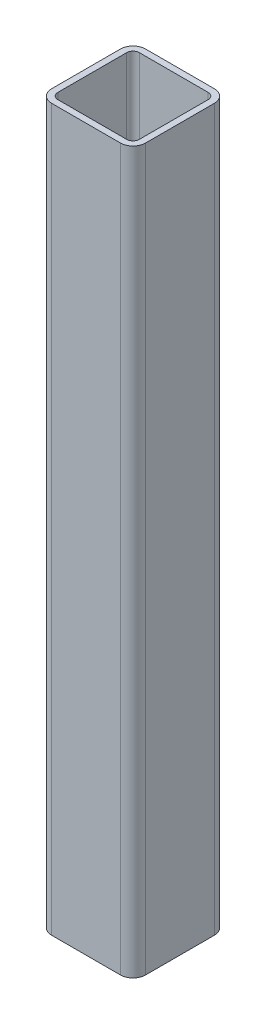
SolidWorks part; units mm, degrees
material "Q235B"
ref_plane "Front Plane" through (0, 0, 0) normal (0, 0, 1) x (1, 0, 0)
ref_plane "Top Plane" through (0, 0, 0) normal (0, 1, 0) x (1, 0, 0)
ref_plane "Right Plane" through (0, 0, 0) normal (1, 0, 0) x (0, 0, -1)
sketch "Sketch1" plane through (0, 0, 0) normal (0, 0, 1) x (1, 0, 0)
  line L0 (0, 0) -> (0, 230)
  dimension "D1" = 230
other "Gb／t 6728—2002 square hollow section 30×30×2(1)"
ref_plane "Plane1" through (0, 0, 0) normal (0, 1, 0) x (-1, 0, 0)
sketch "Sketch11" plane through (0, 0, 0) normal (0, 1, 0) x (-1, 0, 0)
  line L0 (-11, -13) -> (11, -13)
  line L1 (-13, -11) -> (-13, 11)
  line L2 (11, 13) -> (-11, 13)
  line L3 (13, 11) -> (13, -11)
  line L4 (-11, -15) -> (11, -15)
  line L5 (-15, -11) -> (-15, 11)
  line L6 (11, 15) -> (-11, 15)
  line L7 (15, 11) -> (15, -11)
  arc A0 (15, 11) -> (11, 15) centre (11, 11) ccw
  arc A1 (11, -15) -> (15, -11) centre (11, -11) ccw
  arc A2 (-15, -11) -> (-11, -15) centre (-11, -11) ccw
  arc A3 (-11, 15) -> (-15, 11) centre (-11, 11) ccw
  arc A4 (-11, 13) -> (-13, 11) centre (-11, 11) ccw
  arc A5 (13, 11) -> (11, 13) centre (11, 11) ccw
  arc A6 (11, -13) -> (13, -11) centre (11, -11) ccw
  arc A7 (-13, -11) -> (-11, -13) centre (-11, -11) ccw
  point P0 (-15, 0)
  point P1 (15, 0)
  point P2 (0, 15)
  point P3 (0, -15)
  point P4 (0, 0)
  point P5 (-15, -15)
  point P6 (15, -15)
  point P7 (15, 15)
  point P8 (-15, 15)
  point P33 (0, 0)
  dimension "D1" = 4
  dimension "Thickness" = 2
  dimension "V_leg" = 30
